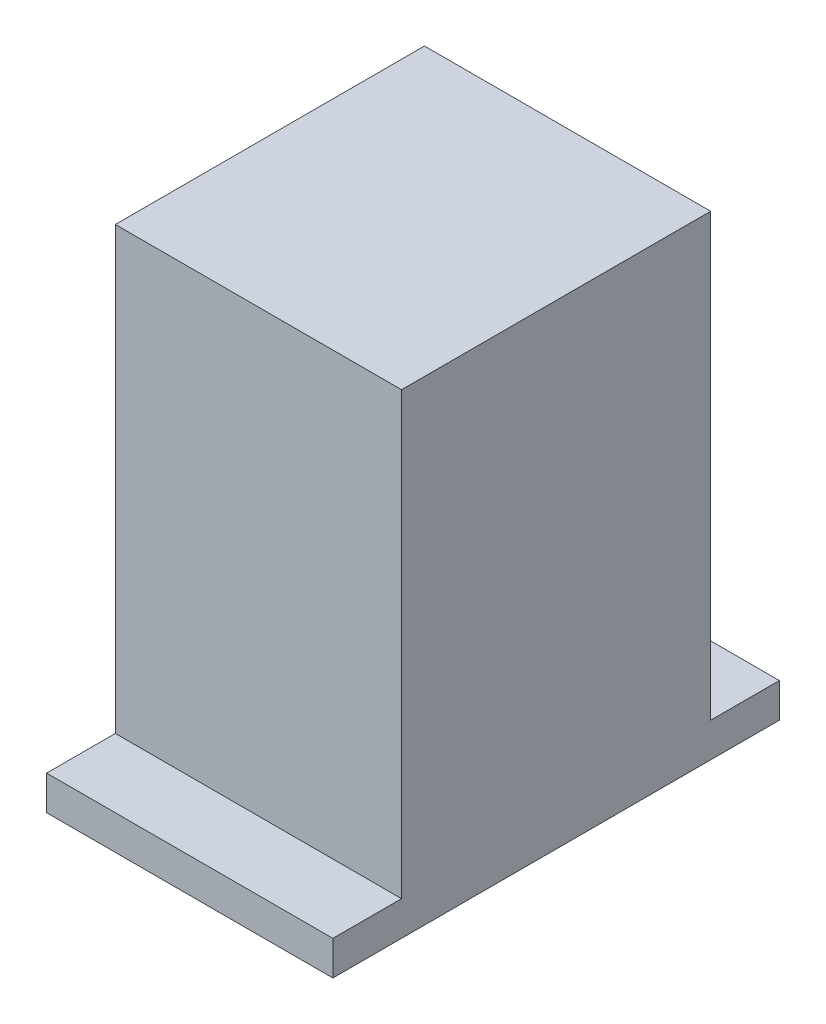
SolidWorks part; units mm, degrees
material "Q235A"
ref_plane "Front Plane" through (0, 0, 0) normal (0, 0, 1) x (1, 0, 0)
ref_plane "Top Plane" through (0, 0, 0) normal (0, 1, 0) x (1, 0, 0)
ref_plane "Right Plane" through (0, 0, 0) normal (1, 0, 0) x (0, 0, -1)
sketch "Sketch1" plane through (0, 0, 0) normal (0, 0, 1) x (1, 0, 0)
  line L1 (25, -41.5) -> (-25, -41.5)
  line L2 (25, -41.5) -> (25, 41.5)
  line L3 (25, 41.5) -> (-25, 41.5)
  line L4 (-25, -41.5) -> (-25, 41.5)
  line L5 (25, -41.5) -> (-25, 41.5) construction
  line L6 (25, 41.5) -> (-25, -41.5) construction
  point P0 (0, 0)
  dimension "D1" = 50
  dimension "D2" = 83
extrude "Boss-Extrude1" add sketch "Sketch1" along normal mid plane 78
sketch "Sketch2" plane through (-25, 0, 0) normal (-1, 0, 0) x (0, 0, 1)
  line L0 (0, -41.5) -> (0, 46.7483) construction
  line L1 (-39, 41.5) -> (-27, 41.5)
  line L2 (-39, 41.5) -> (-39, -35.5)
  line L3 (-39, -35.5) -> (-27, -35.5)
  line L4 (-27, 41.5) -> (-27, -35.5)
  line L5 (39, -41.5) -> (-39, -41.5) construction
  line L6 (27, 41.5) -> (27, -35.5)
  line L7 (39, -35.5) -> (27, -35.5)
  line L8 (39, 41.5) -> (39, -35.5)
  line L9 (39, 41.5) -> (27, 41.5)
  dimension "D1" = 12
  dimension "D2" = 77
extrude "Cut-Extrude1" cut sketch "Sketch2" against normal through all
